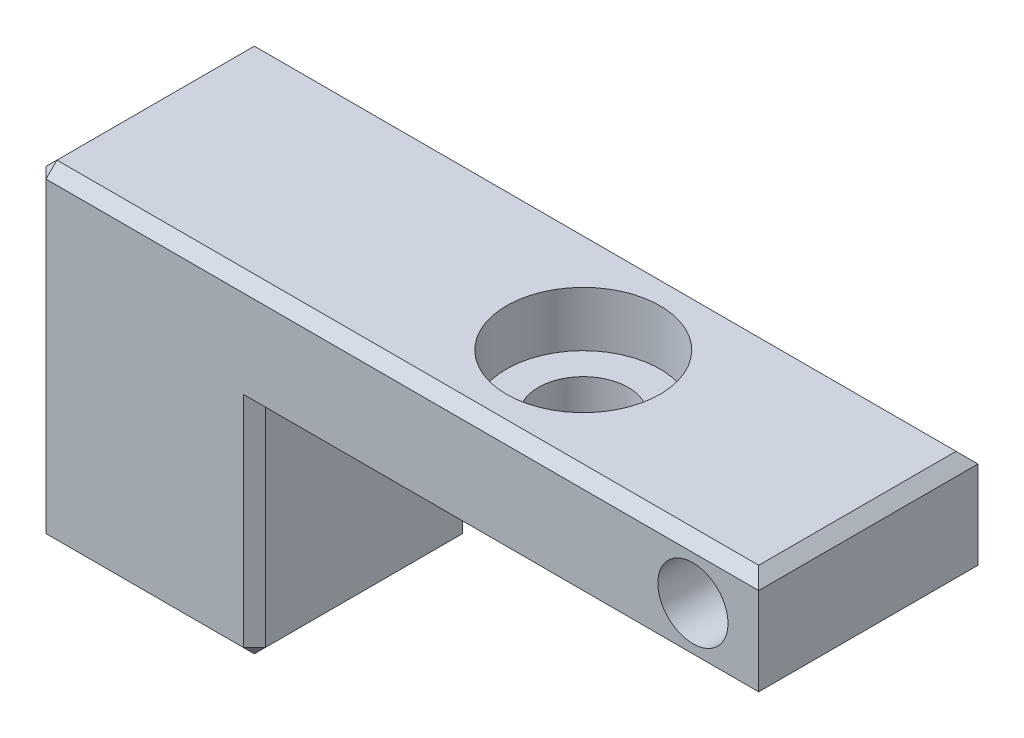
SolidWorks part; units mm, degrees
material "A6061"
ref_plane "Front Plane" through (0, 0, 0) normal (0, 0, 1) x (1, 0, 0)
ref_plane "Top Plane" through (0, 0, 0) normal (0, 1, 0) x (1, 0, 0)
ref_plane "Right Plane" through (0, 0, 0) normal (1, 0, 0) x (0, 0, -1)
sketch "Sketch1" plane through (0, 0, 0) normal (0, 0, 1) x (1, 0, 0)
  line L1 (-16.5, -7.5) -> (16.5, -7.5)
  line L2 (-16.5, -7.5) -> (-16.5, 7.5)
  line L3 (-16.5, 7.5) -> (16.5, 7.5)
  line L4 (16.5, -7.5) -> (16.5, 7.5)
  line L5 (-16.5, -7.5) -> (16.5, 7.5) construction
  line L6 (-16.5, 7.5) -> (16.5, -7.5) construction
  point P0 (0, 0)
  dimension "D1" = 33
  dimension "D2" = 15
extrude "Boss-Extrude1" add sketch "Sketch1" along normal blind 10
sketch "Sketch2" plane through (0, 0, 10) normal (0, 0, 1) x (1, 0, 0)
  line L0 (16.5, 7.5) -> (-16.5, 7.5) construction
  line L1 (16.5, -7.5) -> (-6.5, -7.5)
  line L2 (16.5, -7.5) -> (16.5, 2.5)
  line L3 (16.5, 2.5) -> (-6.5, 2.5)
  line L4 (-6.5, -7.5) -> (-6.5, 2.5)
  line L5 (-16.5, 7.5) -> (-16.5, -7.5) construction
  dimension "D1" = 5
  dimension "D2" = 10
extrude "Cut-Extrude1" cut sketch "Sketch2" against normal blind 20
hole_wizard "M4 Tapped Hole1" positions "Sketch4" profile "Sketch3" tap size "M4" standard "GB"
sketch "Sketch4" plane through (0, -7.5, 0) normal (0, -1, 0) x (-1, 0, 0)
  line L0 (16.5, -10) -> (16.5, 0) construction
  line L1 (16.5, -10) -> (6.5, -10) construction
  point P0 (11.5, -5)
  dimension "D1" = 5
  dimension "D2" = 5
sketch "Sketch3" plane through (-11.5, -7.5, 5) normal (1, 0, 0) x (0, 0, -1)
  line L0 (0, 0) -> (0, 11.0914)
  line L1 (0, 11.0914) -> (1.65, 10.1)
  line L2 (1.65, 10.1) -> (1.65, 0)
  line L5 (1.65, 0) -> (0, 0)
  line L10 (0, 11.0914) -> (-1.65, 10.1) construction
  line L11 (0, -6.35) -> (0, 107.95) construction
  dimension "螺纹孔钻头直径" = 3.3
  dimension "螺纹孔钻头深度" = 10.1
  dimension "导头角度" = 118
cosmetic thread "Cosmetic Thread1" parameters "D1"=8, "D2"=4
sketch "Sketch5" plane through (0, 7.5, 0) normal (0, 1, 0) x (1, 0, 0)
  line L0 (13.5, -5) -> (3.5, -5) construction
  line L1 (13.5, -7.25) -> (3.5, -7.25)
  line L2 (13.5, -2.75) -> (3.5, -2.75)
  line L3 (16.5, -10) -> (16.5, 0) construction
  line L4 (16.5, -10) -> (-16.5, -10) construction
  arc A0 (13.5, -7.25) -> (13.5, -2.75) centre (13.5, -5) ccw
  arc A1 (3.5, -2.75) -> (3.5, -7.25) centre (3.5, -5) ccw
  point P2 (8.5, -5)
  dimension "D1" = 10
  dimension "D2" = 3
  dimension "D3" = 4.5
  dimension "D4" = 5
extrude "Cut-Extrude2" [suppressed] cut sketch "Sketch5" against normal through all
chamfer "Chamfer1" distance 0.5 angle 45 15 edges at (0, 7.5, 10) (16.5, 7.5, 5) (0, 7.5, 0) (16.5, 2.5, 5) (5, 2.5, 0) (5, 2.5, 10) (-16.5, 7.5, 5) (-6.5, -2.5, 10) (-6.5, -2.5, 0) (-11.5, -7.5, 0) (-6.5, -7.5, 5) (-11.5, -7.5, 10) (-16.5, 0, 10) (-16.5, -7.5, 5) (-16.5, 0, 0)
sketch "Sketch6" plane through (0, 7.5, 0) normal (0, 1, 0) x (1, 0, 0)
  line L1 (16.5, 0) -> (-16.5, 0) construction
  line L2 (-16.5, -10) -> (-16.5, 0) construction
  circle A0 centre (3.5, -5) radius 3.5
  dimension "D1" = 7
  dimension "D2" = 20
  dimension "D3" = 5
extrude "Cut-Extrude3" cut sketch "Sketch6" against normal blind 2.5
sketch "Sketch7" plane through (0, 0, 0) normal (0, 0, -1) x (-1, 0, 0)
  line L0 (-16.5, 3) -> (-16.5, 7) construction
  circle A0 centre (-13.5, 5) radius 1.6
  dimension "D1" = 3.2
  dimension "D2" = 3
extrude "Cut-Extrude4" cut sketch "Sketch7" against normal blind 3
ref_plane "Plane1" through (0, 0, 5) normal (0, 0, -1) x (-1, 0, 0)
mirror "Mirror1" about plane through (0, 0, 5) normal (0, 0, -1) of "Cut-Extrude4"
sketch "Sketch8" plane through (0, 5, 0) normal (0, 1, 0) x (1, 0, 0)
  circle A0 centre (3.5, -5) radius 2.05
  dimension "D1" = 4.1
extrude "Cut-Extrude5" cut sketch "Sketch8" against normal blind 10
